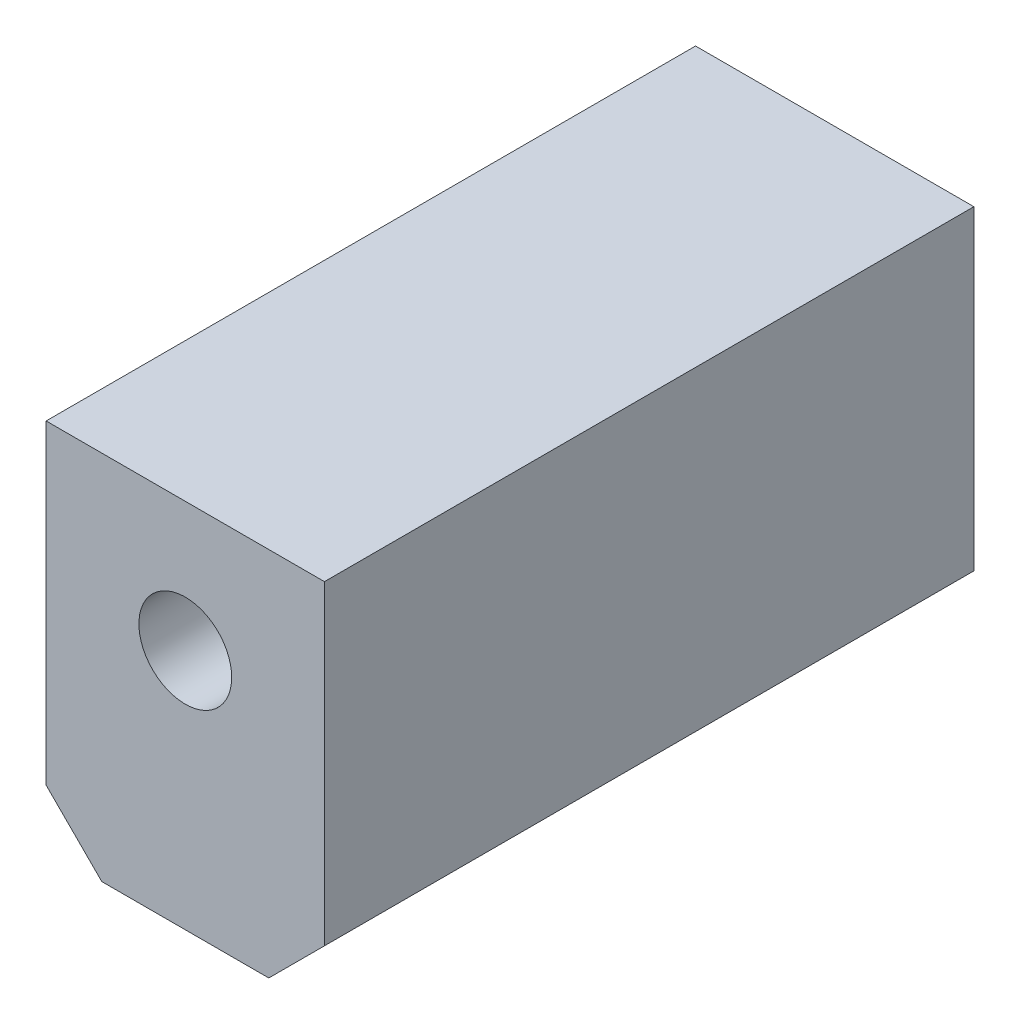
from build123d import *

# Parameters (mm, degrees)
SKETCH1_W             = 15
SKETCH1_H             = 20
BOSS_EXTRUDE1_DEPTH   = 17.5
CHAMFER1_SIZE         = 3
M6_TAPPED_HOLE1_D     = 5
M6_TAPPED_HOLE1_DEPTH = 15
M6_TAPPED_HOLE1_TIP   = 1.502151548


with BuildPart() as part:
    # Sketch1 → Boss-Extrude1 (new, symmetric)
    with BuildSketch(Plane.XY):
        Rectangle(SKETCH1_W, SKETCH1_H)
    extrude(amount=BOSS_EXTRUDE1_DEPTH, both=True)

    # Chamfer1
    chamfer1_edges = [part.edges().sort_by_distance(p)[0] for p in [
        (7.5, -10, 0),
        (-7.5, -10, 0),
    ]]
    chamfer(chamfer1_edges, length=CHAMFER1_SIZE)

    # M6 Tapped Hole1
    with Locations(Plane.XY.offset(17.5)):
        with Locations((0, 3.03)):
            Hole(M6_TAPPED_HOLE1_D / 2, depth=M6_TAPPED_HOLE1_DEPTH)
            with Locations((0, 0, -(M6_TAPPED_HOLE1_DEPTH + M6_TAPPED_HOLE1_TIP / 2))):  # 118° drill point
                Cone(0, M6_TAPPED_HOLE1_D / 2, M6_TAPPED_HOLE1_TIP, mode=Mode.SUBTRACT)


solid = part.part
